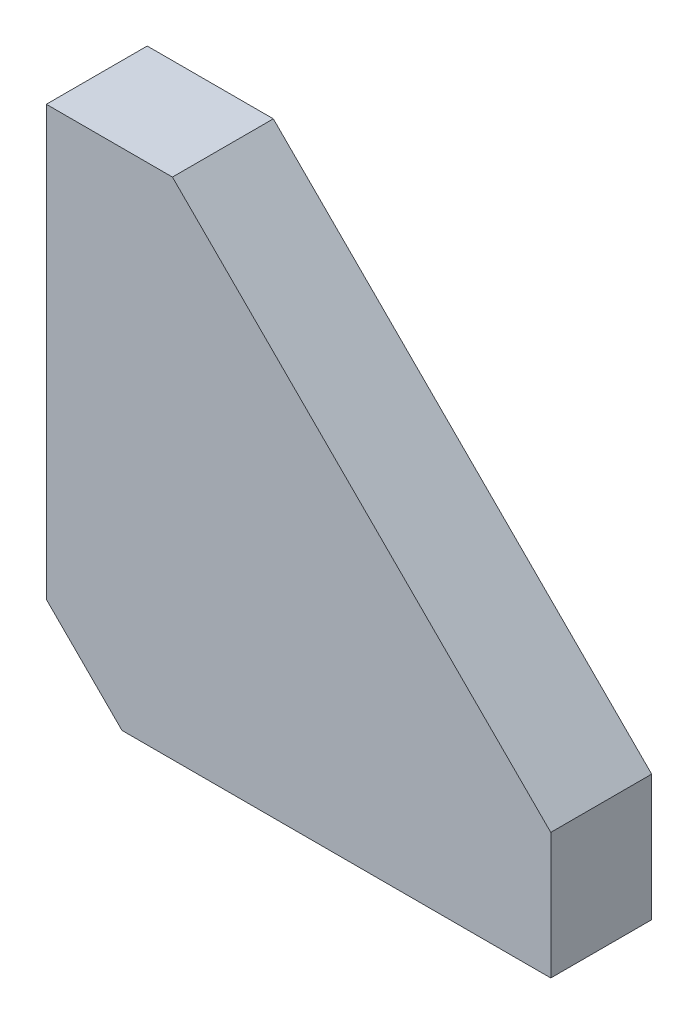
from build123d import *

# Parameters (mm, degrees)
BOSS_EXTRUDE1_DEPTH = 20
CHAMFER1_SIZE       = 15


with BuildPart() as part:
    # Sketch1 → Boss-Extrude1 (new body)
    with BuildSketch(Plane.XY):
        Polygon((0, 0), (100, 0), (100, 25), (25, 100), (0, 100), align=None)
    extrude(amount=BOSS_EXTRUDE1_DEPTH)

    # Chamfer1
    chamfer1_edges = [part.edges().sort_by_distance(p)[0] for p in [
        (0, 0, 10),
    ]]
    chamfer(chamfer1_edges, length=CHAMFER1_SIZE)


solid = part.part
